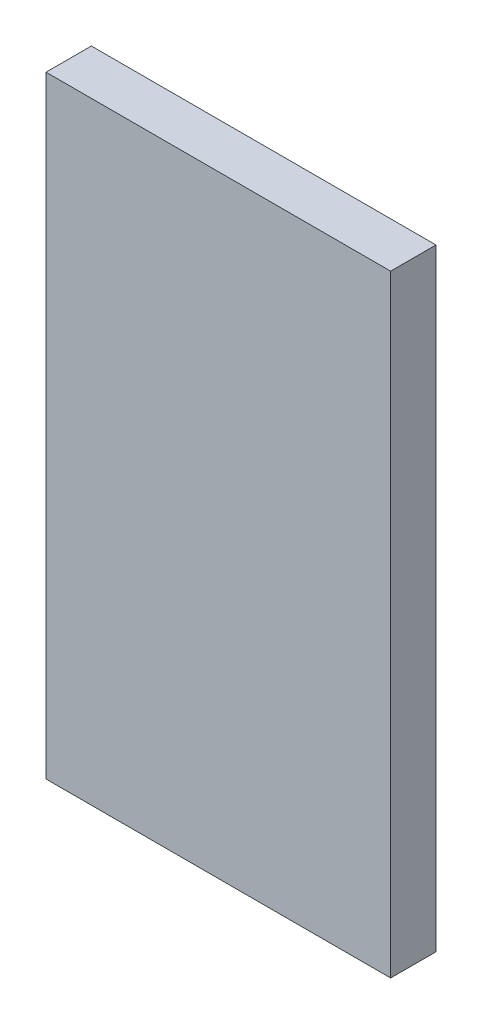
SolidWorks part; units mm, degrees
ref_plane "Front Plane" through (0, 0, 0) normal (0, 0, 1) x (1, 0, 0)
ref_plane "Top Plane" through (0, 0, 0) normal (0, 1, 0) x (1, 0, 0)
ref_plane "Right Plane" through (0, 0, 0) normal (1, 0, 0) x (0, 0, -1)
other "Configuration Table"
sketch "Sketch1" plane through (0, 0, 0) normal (0, 0, 1) x (1, 0, 0)
  line L1 (0, 0) -> (152, 0)
  line L2 (0, 0) -> (0, 270)
  line L3 (0, 270) -> (152, 270)
  line L4 (152, 0) -> (152, 270)
  dimension "D1" = 152
  dimension "D2" = 270
extrude "Boss-Extrude1" add sketch "Sketch1" along normal blind 20
